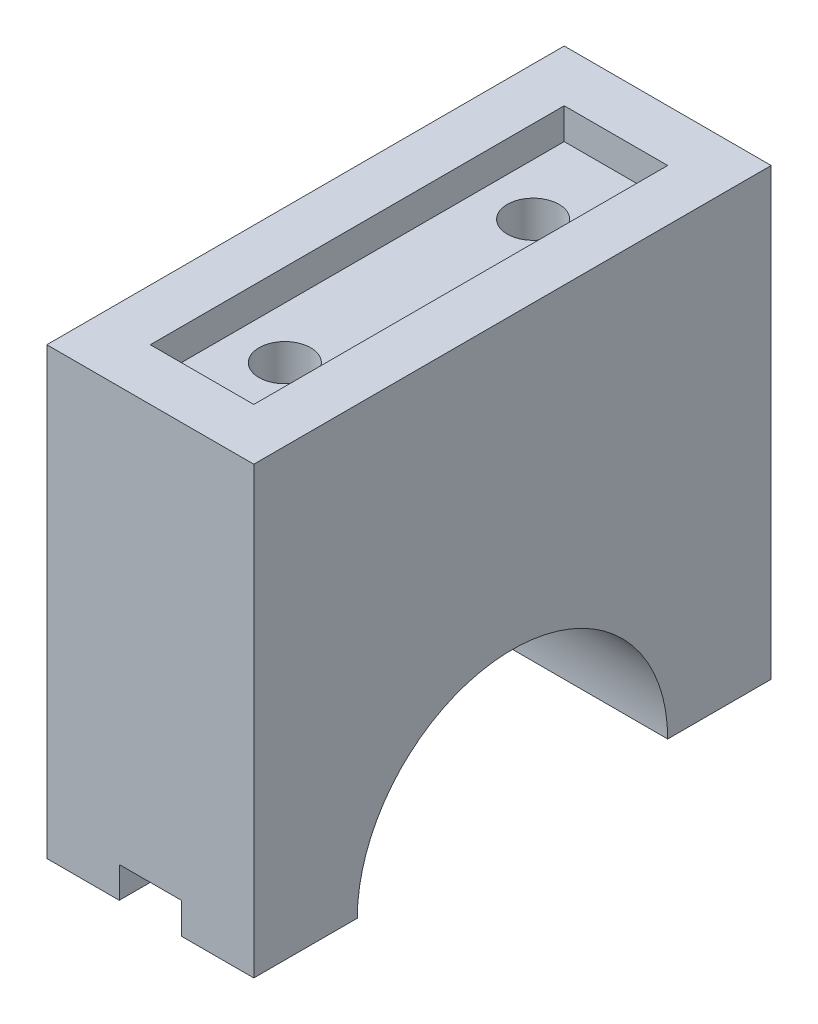
SolidWorks part; units mm, degrees
ref_plane "Front Plane" through (0, 0, 0) normal (0, 0, 1) x (1, 0, 0)
ref_plane "Top Plane" through (0, 0, 0) normal (0, 1, 0) x (1, 0, 0)
ref_plane "Right Plane" through (0, 0, 0) normal (1, 0, 0) x (0, 0, -1)
sketch "Sketch1" plane through (0, 0, 0) normal (0, 0, 1) x (1, 0, 0)
  line L1 (10, 21.5) -> (-10, 21.5)
  line L2 (10, 21.5) -> (10, -21.5)
  line L3 (10, -21.5) -> (-10, -21.5)
  line L4 (-10, 21.5) -> (-10, -21.5)
  line L5 (10, 21.5) -> (-10, -21.5) construction
  line L6 (10, -21.5) -> (-10, 21.5) construction
  point P0 (0, 0)
  dimension "D1" = 20
  dimension "D2" = 43
extrude "Boss-Extrude1" add sketch "Sketch1" along normal blind 50
sketch "Sketch2" plane through (10, 0, 0) normal (1, 0, 0) x (0, 0, -1)
  line L0 (-50, -21.5) -> (0, -21.5) construction
  circle A0 centre (-25, -21.5) radius 15
  dimension "D1" = 30
extrude "Cut-Extrude1" cut sketch "Sketch2" against normal blind 50
sketch "Sketch3" plane through (-10, 0, 0) normal (-1, 0, 0) x (0, 0, 1)
  line L0 (19.0839, -4.5) -> (30.9161, -4.5)
  line L1 (50, -21.5) -> (40, -21.5) construction
  arc A0 (19.0839, -4.5) -> (30.9161, -4.5) centre (25, -21.5) ccw
  dimension "D1" = 36
  dimension "D2" = 17
extrude "Cut-Extrude2" cut sketch "Sketch3" against normal blind 5
sketch "Sketch4" plane through (0, -21.5, 0) normal (0, -1, 0) x (1, 0, 0)
  line L0 (-5, 25) -> (-13.5793, 25) construction
  line L1 (-3, 5) -> (3, 5)
  line L2 (-3, 5) -> (-3, 0)
  line L3 (-3, 0) -> (3, 0)
  line L4 (3, 5) -> (3, 0)
  line L5 (-3, 5) -> (3, 0) construction
  line L6 (-3, 0) -> (3, 5) construction
  line L7 (-5, 40) -> (-5, 10) construction
  line L8 (-10, 0) -> (10, 0) construction
  line L9 (-3, 50) -> (3, 45) construction
  line L10 (-3, 45) -> (3, 50) construction
  line L11 (3, 45) -> (3, 50)
  line L12 (-3, 50) -> (3, 50)
  line L13 (-3, 45) -> (-3, 50)
  line L14 (-3, 45) -> (3, 45)
  point P0 (0, 2.5)
  point P17 (0, 47.5)
  dimension "D1" = 6
  dimension "D2" = 5
extrude "Cut-Extrude3" cut sketch "Sketch4" against normal blind 3
sketch "Sketch5" plane through (0, -21.5, 0) normal (0, -1, 0) x (1, 0, 0)
  line L0 (3, 0) -> (10, 0) construction
  line L1 (-10, 7) -> (-10, 0) construction
  line L2 (-10, 25) -> (0, 25) construction
  line L3 (-10, 30.9161) -> (-10, 19.0839) construction
  circle A0 centre (-6, 4) radius 2
  circle A2 centre (6, 4) radius 2
  circle A3 centre (6, 46) radius 2
  circle A4 centre (-6, 46) radius 2
  dimension "D4" = 4
  dimension "D1" = 12
  dimension "D2" = 4
  dimension "D3" = 4
hole_wizard "Size mm Dowel hole 1" positions "Sketch6" profile "Sketch7" hole size "Ø12.0" standard "GB"
sketch "Sketch6" plane through (0, -21.5, 0) normal (0, -1, 0) x (-1, 0, 0)
  point P0 (6, -4)
  point P3 (-6, -4)
  point P7 (6, -46)
  point P10 (-6, -46)
sketch "Sketch7" plane through (-6, -21.5, 4) normal (1, 0, 0) x (0, 0, -1)
  line L0 (0, 0) -> (0, 15.4618)
  line L1 (0, 15.4618) -> (2.1, 14.2)
  line L2 (2.1, 14.2) -> (2.1, 0)
  line L5 (2.1, 0) -> (0, 0)
  line L10 (0, 15.4618) -> (-2.1, 14.2) construction
  line L11 (0, -6.35) -> (0, 107.95) construction
  dimension "孔直径" = 4.2
  dimension "孔深度" = 14.2
  dimension "导头角度" = 118
sketch "Sketch8" plane through (0, 21.5, 0) normal (0, 1, 0) x (1, 0, 0)
  line L0 (10, -50) -> (10, 0) construction
  line L1 (5, -45) -> (-5, -45)
  line L2 (5, -45) -> (5, -5)
  line L3 (5, -5) -> (-5, -5)
  line L4 (-5, -45) -> (-5, -5)
  line L5 (5, -45) -> (-5, -5) construction
  line L6 (5, -5) -> (-5, -45) construction
  point P0 (0, -25)
  point P8 (10, -25)
  dimension "D1" = 10
  dimension "D2" = 40
extrude "Cut-Extrude4" cut sketch "Sketch8" against normal blind 3
sketch "Sketch9" plane through (0, 18.5, 0) normal (0, 1, 0) x (1, 0, 0)
  circle A0 centre (0, -13) radius 4.0667
  circle A1 centre (0, -37) radius 4.9212
  dimension "D1" = 24
  dimension "D2" = 13
hole_wizard "Size mm Dowel hole 2" positions "Sketch10" profile "Sketch11" hole size "Ø5.0" standard "GB"
sketch "Sketch10" plane through (0, 18.5, 0) normal (0, 1, 0) x (1, 0, 0)
  point P0 (0, -13)
  point P3 (0, -37)
sketch "Sketch11" plane through (0, 18.5, 13) normal (1, 0, 0) x (0, 0, 1)
  line L0 (0, 0) -> (0, 18.6022)
  line L1 (0, 18.6022) -> (2.5, 17.1)
  line L2 (2.5, 17.1) -> (2.5, 0)
  line L5 (2.5, 0) -> (0, 0)
  line L10 (0, 18.6022) -> (-2.5, 17.1) construction
  line L11 (0, -6.35) -> (0, 107.95) construction
  dimension "孔直径" = 5
  dimension "孔深度" = 17.1
  dimension "导头角度" = 118
